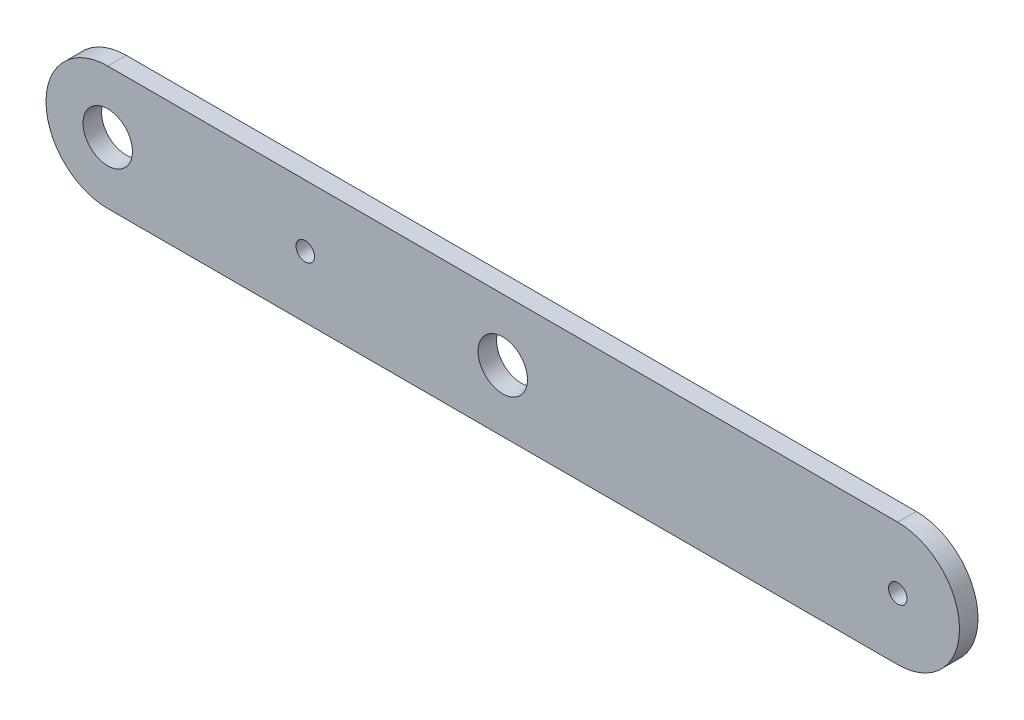
from build123d import *

# Parameters (mm, degrees)
SKETCH_1_R           = 2
SKETCH_1_R_2         = 0.75
BOSS_EXTRUDE_1_DEPTH = 1.5


with BuildPart() as part:
    # Sketch 1 → Boss-Extrude 1 (new body)
    with BuildSketch(Plane.XY):
        with BuildLine():
            Line((-57.299329586, 5), (6.700670414, 5))
            ThreePointArc((6.700670414, 5), (11.700670414, 0), (6.700670414, -5))
            Line((6.700670414, -5), (-57.299329586, -5))
            ThreePointArc((-57.299329586, -5), (-62.299329586, 0), (-57.299329586, 5))
        make_face()
        with Locations((-57.299329586, 0)):
            Circle(SKETCH_1_R, mode=Mode.SUBTRACT)
        with Locations((6.700670414, 0)):
            Circle(SKETCH_1_R_2, mode=Mode.SUBTRACT)
        with Locations((-41.299329586, 0)):
            Circle(SKETCH_1_R_2, mode=Mode.SUBTRACT)
        with Locations((-25.299329586, 0)):
            Circle(SKETCH_1_R, mode=Mode.SUBTRACT)
    extrude(amount=BOSS_EXTRUDE_1_DEPTH)


solid = part.part
